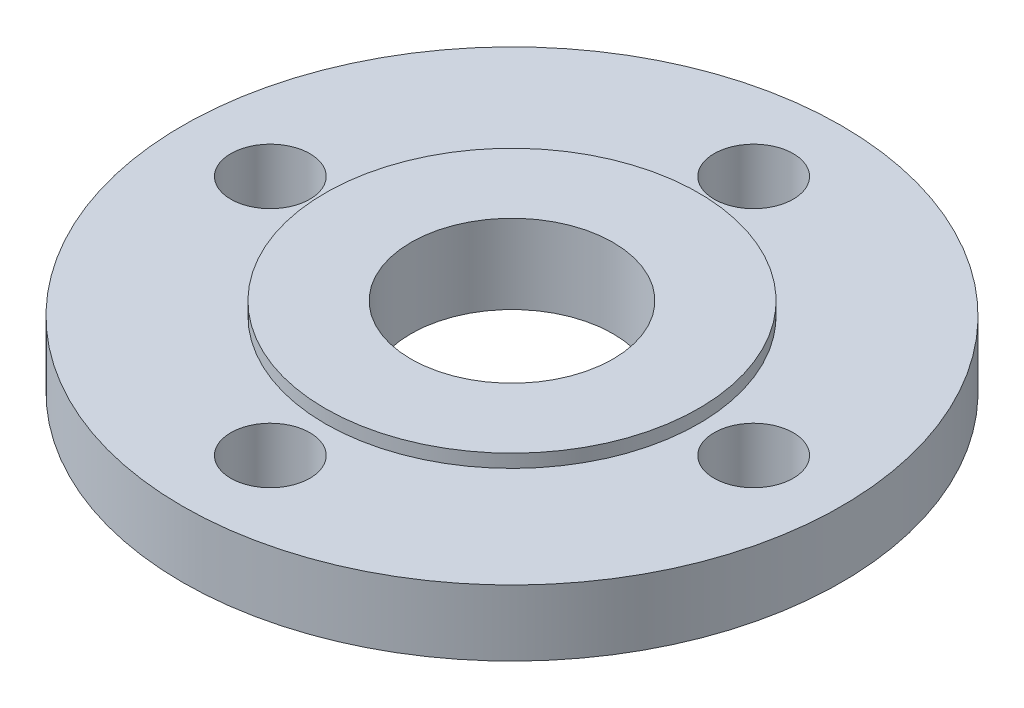
SolidWorks part; units mm, degrees
ref_plane "Front" through (0, 0, 0) normal (0, 0, 1) x (1, 0, 0)
ref_plane "Top" through (0, 0, 0) normal (0, 1, 0) x (1, 0, 0)
ref_plane "Right" through (0, 0, 0) normal (1, 0, 0) x (0, 0, -1)
sketch "草图1" plane through (0, 0, 0) normal (0, 1, 0) x (1, 0, 0)
  circle A0 centre (0, 0) radius 75
  circle A1 centre (0, 0) radius 55 construction
  circle A2 centre (0, 55) radius 9
  circle A3 centre (55, 0) radius 9
  circle A4 centre (0, -55) radius 9
  circle A5 centre (-55, 0) radius 9
  circle A6 centre (0, 0) radius 23
  point P15 (0, 0)
  dimension "D1" = 150
  dimension "D2" = 110
  dimension "D3" = 18
  dimension "D5" = 46
  dimension "D4" = 4
extrude "凸台-拉伸1" add sketch "草图1" along normal blind 15
sketch "草图2" plane through (0, 15, 0) normal (0, 1, 0) x (1, 0, 0)
  circle A0 centre (0, 0) radius 42.5
  circle A1 centre (0, 0) radius 23
  dimension "D1" = 85
extrude "凸台-拉伸2" add sketch "草图2" along normal blind 3
